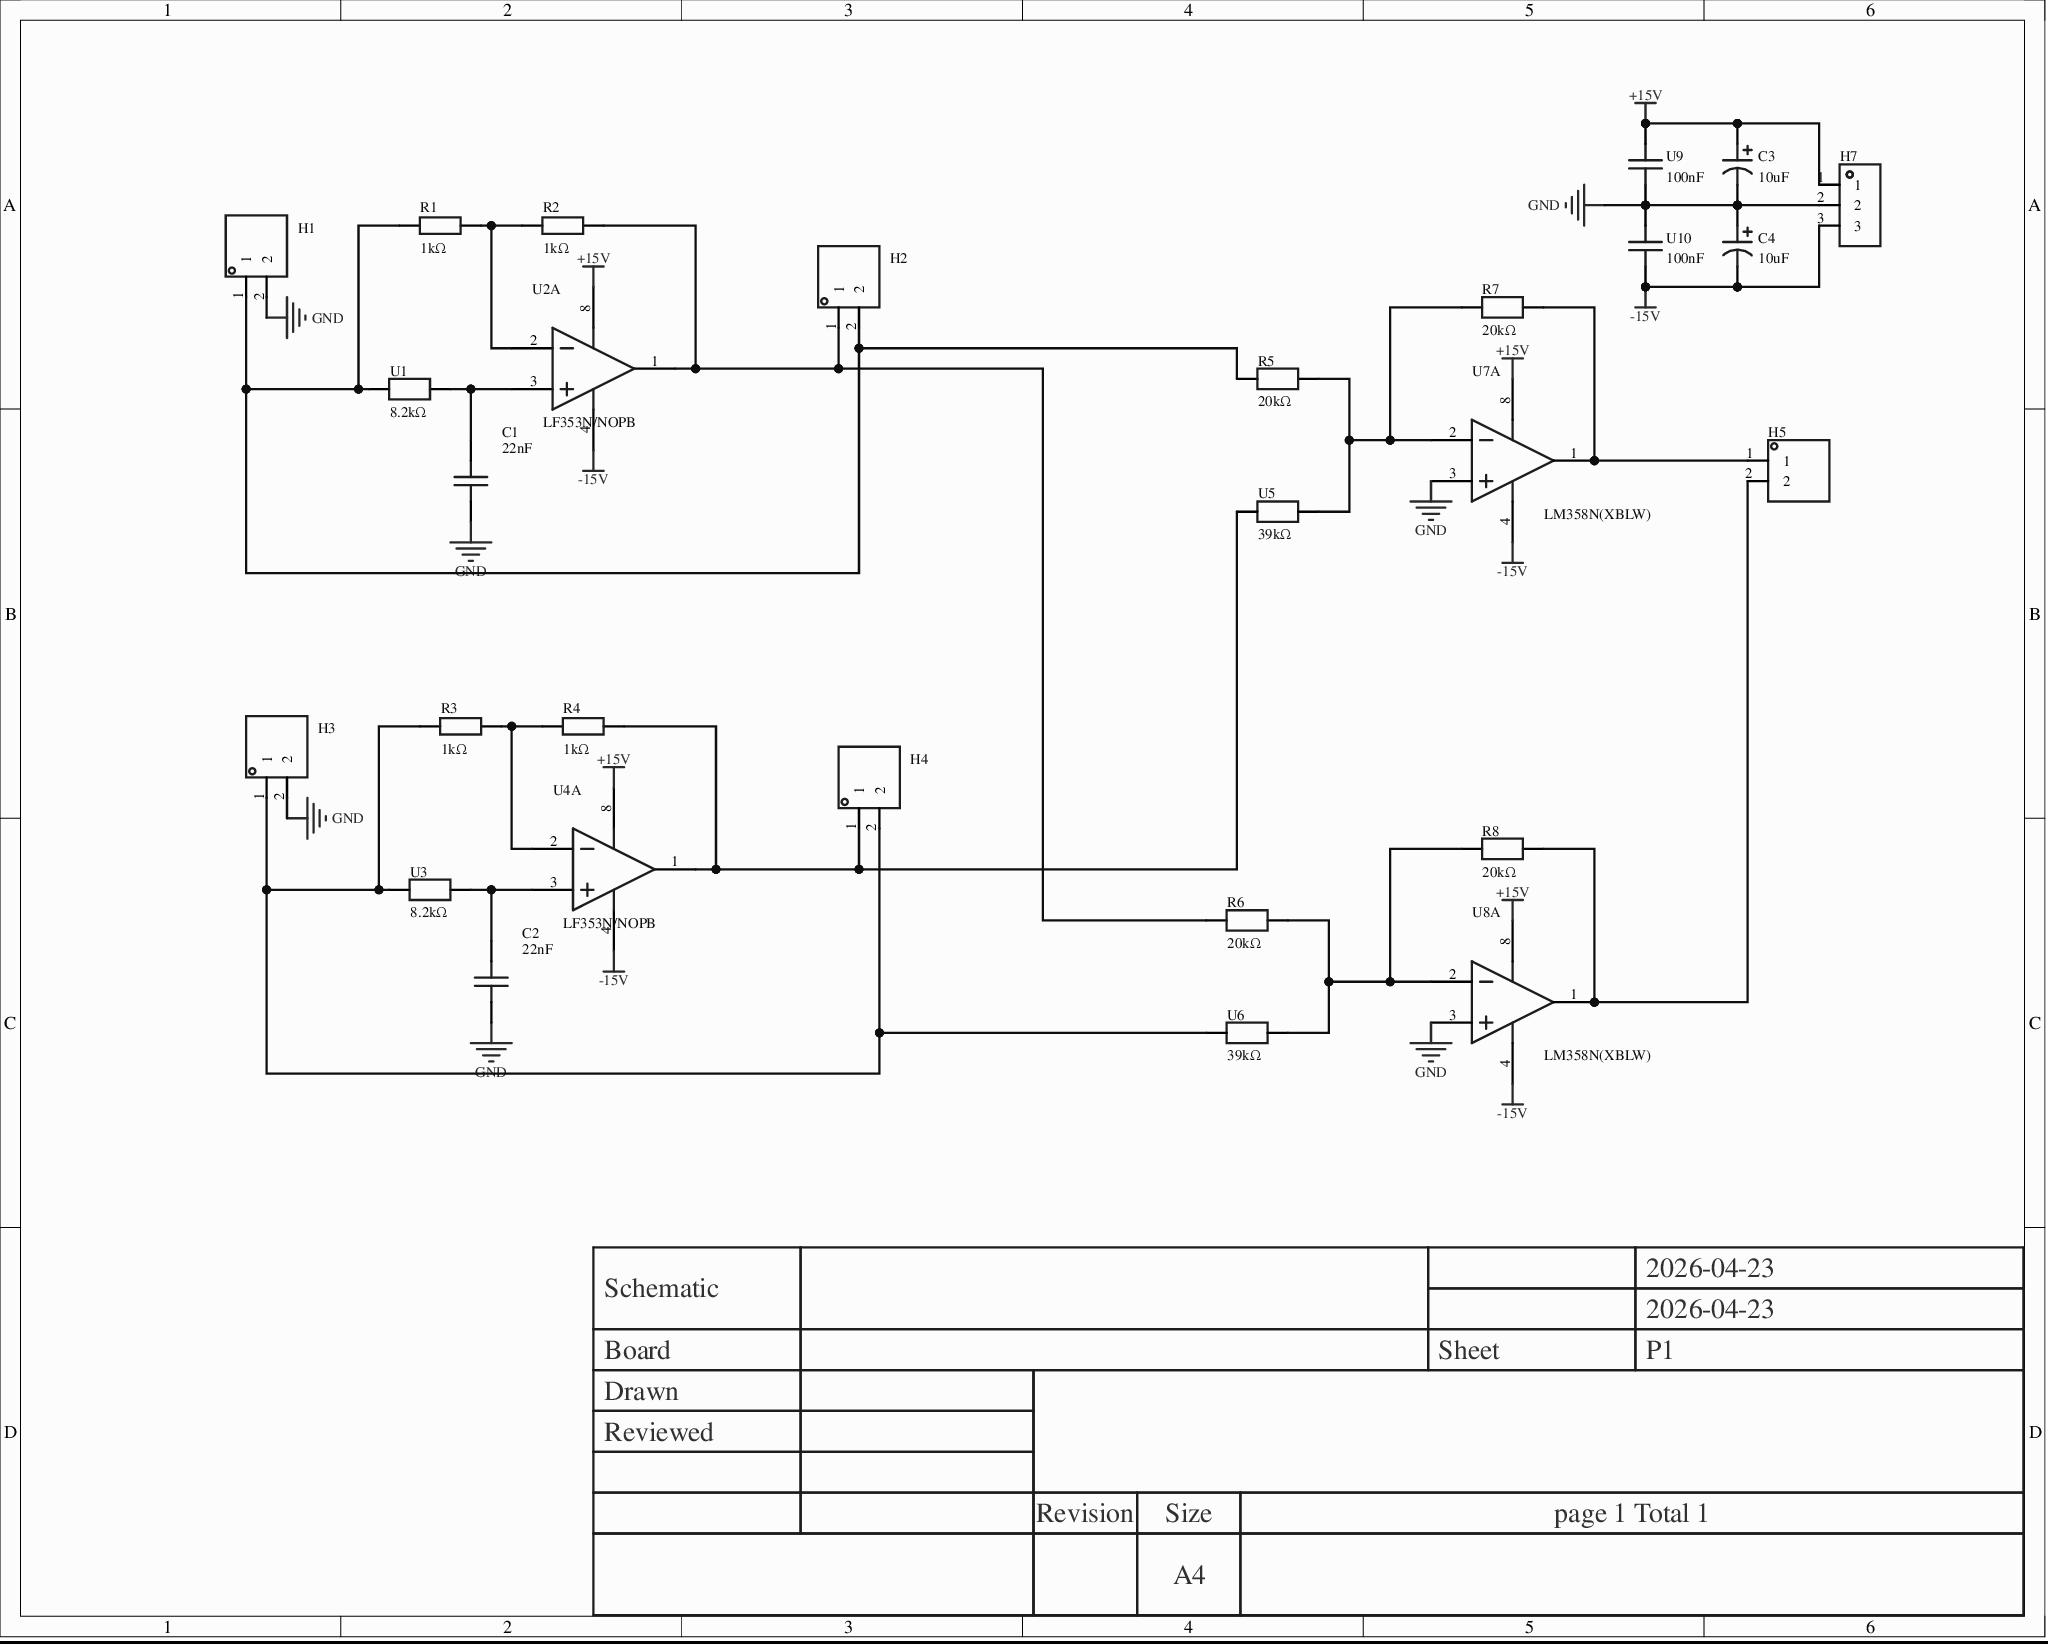
[diagram p0: MISC49900-3.schdoc]
# Altium project MISC49900-2.PrjPcb
1 sheet, 28 parts. Net scope: global (net labels, ports and power ports of the same name join across sheets).
Board file: MISC49900.pcbdoc

## Sheet MISC49900-3.schdoc
size 254 x 203 mm; Version: V1.0; @Project Name: MISC49900; @Update Date: 2026-04-26; @Create Date: 2026-04-26; @Board Name: MISC49900; @Create Time: 22:45:20; @Page Count: 1; @Page No: 1; @Schematic Name: MISC49900; @Update Time: 22:45:20; Size: A4

### Parts
C1  22nF  [CAP-TH_L12.0-W4.5-P10.00-D1.0]
C2  22nF  [CAP-TH_L12.0-W4.5-P10.00-D1.0]
C3  10uF  [CAP-TH_BD5.0-P2.00-D0.8-FD-10UF50VC110GL]
C4  10uF  [CAP-TH_BD5.0-P2.00-D0.8-FD-10UF50VC110GL]
H1  (no value)  [HDR-TH_2P-P2.54-V-M-1]
H2  (no value)  [HDR-TH_2P-P2.54-V-M-1]
H3  (no value)  [HDR-TH_2P-P2.54-V-M-1]
H4  (no value)  [HDR-TH_2P-P2.54-V-M-1]
H5  (no value)  [HDR-TH_2P-P2.54-V-M-1]
H7  (no value)  [HDR-TH_3P-P2.54-V-M]
R1  1kΩ  [RES-TH_BD2.5-L6.5-P10.50-D0.6]
R2  1kΩ  [RES-TH_BD2.5-L6.5-P10.50-D0.6]
R3  1kΩ  [RES-TH_BD2.5-L6.5-P10.50-D0.6]
R4  1kΩ  [RES-TH_BD2.5-L6.5-P10.50-D0.6]
R5  20kΩ  [RES-TH_BD2.4-L6.3-P10.30-D0.6]
R6  20kΩ  [RES-TH_BD2.4-L6.3-P10.30-D0.6]
R7  20kΩ  [RES-TH_BD2.4-L6.3-P10.30-D0.6]
R8  20kΩ  [RES-TH_BD2.4-L6.3-P10.30-D0.6]
U1  8.2kΩ  [RES-TH_BD2.7-L6.2-P10.20-D0.4]
U2  LF353N/NOPB  [PDIP-8_L9.6-W6.4-P2.54-LS7.6-BL]  (part A of 2)
U3  8.2kΩ  [RES-TH_BD2.7-L6.2-P10.20-D0.4]
U4  LF353N/NOPB  [PDIP-8_L9.6-W6.4-P2.54-LS7.6-BL]  (part A of 2)
U5  39kΩ  [RES-TH_BD2.4-L6.3-P10.30-D0.6]
U6  39kΩ  [RES-TH_BD2.4-L6.3-P10.30-D0.6]
U7  LM358N(XBLW)  [PDIP-8_L9.3-W6.4-P2.54-LS7.6-BL]  (part A of 2)
U8  LM358N(XBLW)  [PDIP-8_L9.3-W6.4-P2.54-LS7.6-BL]  (part A of 2)
U9  100nF  [CAP-TH_L5.0-W2.5-P5.00-D1.0]
U10  100nF  [CAP-TH_L5.0-W2.5-P5.00-D1.0]

### Nets
+15V: C3.1 H7.1 U2.8(VCC) U4.8(VCC) U7.8(V+) U8.8(V+) U9.1
-15V: C4.2 H7.3 U2.4(VEE) U4.4(VEE) U7.4(V-) U8.4(V-) U10.2
GND: C1.1 C2.1 C3.2 C4.1 H1.2 H3.2 H7.2 U7.3(IN_A+) U8.3(IN_A+) U9.2 U10.1
NetC1_2: C1.2 U1.2 U2.3(INA+)
NetC2_2: C2.2 U3.2 U4.3(INA+)
NetH1_1: H1.1 H2.2 R1.1 R5.1 U1.1
NetH2_1: H2.1 R2.2 R6.1 U2.1(OUTA)
NetH3_1: H3.1 H4.2 R3.1 U3.1 U6.1
NetH4_1: H4.1 R4.2 U4.1(OUTA) U5.1
NetH5_1: H5.1 R7.2 U7.1(OUT_A)
NetH5_2: H5.2 R8.2 U8.1(OUT_A)
NetR1_2: R1.2 R2.1 U2.2(INA-)
NetR3_2: R3.2 R4.1 U4.2(INA-)
NetR5_2: R5.2 R7.1 U5.2 U7.2(IN_A-)
NetR6_2: R6.2 R8.1 U6.2 U8.2(IN_A-)

### Notes on the sheet
- 2026-04-23
- Schematic
- Board
- Sheet
- P1
- Drawn
- Reviewed
- Revision
- Size
- A4
- page 1 Total 1

### Library data of the parts
C1 C2 = KP223J2J1001: component KP223J2J1001; capacitance: 22nF; tolerance: ±5%; rated voltage: 630V; operating temperature: -40℃~+100℃;; Manufacturer: KYET(科雅); AddInBom: yes; ModelId: 5745697730bf4b0891de41ab4d2b5a300819f05c4eef4c71ace90d822a990e87; ModelName: CAP-TH_L12.0-W4.5-H10.0-P10.0; ModelTransform: 472.44,177.165,0,0,0,0,0,0,-137.795; Device: KP223J2J1001; Symbol: KP223J2J1001; FootprintName: CAP-TH_L12.0-W4.5-P10.00-D1.0; LCSC Part Name: 22nF ±5% 630V; SupplierPart: C390074; ManufacturerPart: KP223J2J1001; Supplier Footprint: 插件,P=10mm; JLCPCB Part Class: Extended Part; Datasheet: example.com/datasheet/KP223J2J1001/366157.html; Supplier: LCSC; ConvertToPcb: yes; Value: 22nF; Tolerance: ±5%; Voltage Rating: 630V; Operating Temperature: -40℃~+100℃
C3 C4 = 10UF50VC110GL: component 10UF50VC110GL; capacitance: 10uF; tolerance: ±20%; rated voltage: 50V; ripple current: 120mA@100KHz; equivalent series resistance (ESR): 1.6Ω;; Manufacturer: Econd(米朗电子); AddInBom: yes; Pin Spacing: 2mm; Lifetime: 5000hrs@105℃; Symbol: 10UF50VC110GL; Device: 10UF50VC110GL; LCSC Part Name: 10uF ±20% 50V; SupplierPart: C46867109; ManufacturerPart: 10UF50VC110GL; Supplier Footprint: 插件,D5xL11mm; JLCPCB Part Class: Extended Part; Datasheet: example.com/datasheet/10UF50VC110GL/49031974.html; Supplier: LCSC; ConvertToPcb: yes; FootprintName: CAP-TH_BD5.0-P2.00-D0.8-FD-10UF50VC110GL; Value: 10uF; Tolerance: ±20%; Voltage Rating: 50V; Ripple Current: 120mA@100KHz; Equivalent Series Resistance(ESR): 1.6Ω; Diameter: 5mm; Height - Seated (Max): 11mm; Operating Temperature: -40℃~+105℃
H1-H5 = HDR-M_2.54_1x2P: Symbol: 210S-1*2P L=11.6MMGold-plated black; ConvertToPcb: yes; ModelId: 79b2e9f2d70a4d68a1b7098f27c6d4c50819f05c4eef4c71ace90d822a990e87; ModelName: HDR-M-2.54_1x2; ModelTransform: 200,100,0,0,0,0,0,0,-118.11; Device: HDR-M_2.54_1x2P; FootprintName: HDR-TH_2P-P2.54-V-M-1; AddInBom: yes; SupplierPart: C124375; Supplier Footprint: 插件
H7 = HDR-M_2.54_1x3P: AddInBom: yes; ModelId: bb473b6d38ff42a99216a4fcdbdcc4cb0819f05c4eef4c71ace90d822a990e87; ModelName: HDR-TH_3P-P2.54-M-LI-1X3P; ModelTransform: 300.03877,100,0,0,0,0,0,0,-118.11; Device: HDR-M_2.54_1x3P; Symbol: HDR-M_2.54_1x3P; FootprintName: HDR-TH_3P-P2.54-V-M; ConvertToPcb: yes; SupplierPart: C2937625; Supplier Footprint: 插件
R1-R4 = MFR0W4F1001A50: component MFR0W4F1001A50; resistor type: metal film resistor; resistance: 1kΩ; tolerance: ±1%; power: 250mW; temperature coefficient: ±50ppm/℃;; Manufacturer: UNI-ROYAL(厚声); AddInBom: yes; Voltage-Supply(Max): 250V; ModelId: 8e6c7ee8323443d1ab8f0504b6353c8c0819f05c4eef4c71ace90d822a990e87; ModelName: RES-TH_D2.3-L6.5-P10.50; ModelTransform: 431.1015,91.3384,0,0,0,0,0.197,0,-137.795; Device: MFR0W4F1001A50; Symbol: MFR0W4F1001A50; FootprintName: RES-TH_BD2.5-L6.5-P10.50-D0.6; LCSC Part Name: 1kΩ ±1% 250mW 金属膜电阻 铜脚，圆柱状直插; SupplierPart: C57435; ManufacturerPart: MFR0W4F1001A50; Supplier Footprint: 插件,D2.2xL6.5mm; JLCPCB Part Class: Extended Part; Datasheet: example.com/20191012/C436293_8820AA14BC71FA35E551C06C441482A0.pdf; Supplier: LCSC; ConvertToPcb: yes; Type: Metal film resistor; Value: 1kΩ; Tolerance: ±1%; Power(Watts): 250mW; Temperature Coefficient: ±50ppm/℃
R5 = RN 1/4W 20K F T/B A1: 电阻类型:金属膜电阻;阻值:20kΩ;精度:±1%;功率:250mW;温度系数:±50ppm/℃;; Manufacturer: Tyohm(幸亚电阻); AddInBom: yes; Tolerance: ±1%; Voltage-Supply(Max): 250V; Power(Watts): 250mW; Description: resistor type: metal film resistor; resistance: 20kΩ; tolerance: ±1%; power: 250mW; temperature coefficient: ±50ppm/℃;; ModelId: 463263665006444ab7a47bd11b0cf9560819f05c4eef4c71ace90d822a990e87; ModelTransform: 427.165,94.32816,0,0,0,0,0,0,-196.85; Device: RN 1/4W 20K F T/B A1; Symbol: RN 1/4W 20K F T/B A1; FootprintName: RES-TH_BD2.4-L6.3-P10.30-D0.6; LCSC Part Name: 20kΩ ±1% 250mW 金属膜电阻; SupplierPart: C410662; ManufacturerPart: RN 1/4W 20K F T/B A1; Supplier Footprint: 插件,D2.4xL6.4mm; JLCPCB Part Class: Extended Part; Datasheet: example.com/datasheet/RN%25201%252F4W%252020K%2520F%2520T%252FB%2520A1/401583.html; Supplier: LCSC; ConvertToPcb: yes; Type: Metal film resistor; Value: 20kΩ; Temperature Coefficient: ±50ppm/℃; Operating Temperature: -55℃~+125℃; ModelName: RES-TH_BD2.4-L6.3-P10.30-D0.6
R6-R8 = RN 1/4W 20K F T/B A1: resistor type: metal film resistor; resistance: 20kΩ; tolerance: ±1%; power: 250mW; temperature coefficient: ±50ppm/℃;; Manufacturer: Tyohm(幸亚电阻); AddInBom: yes; Voltage-Supply(Max): 250V; ModelId: 463263665006444ab7a47bd11b0cf9560819f05c4eef4c71ace90d822a990e87; ModelTransform: 427.165,94.32816,0,0,0,0,0,0,-196.85; Device: RN 1/4W 20K F T/B A1; Symbol: RN 1/4W 20K F T/B A1; FootprintName: RES-TH_BD2.4-L6.3-P10.30-D0.6; LCSC Part Name: 20kΩ ±1% 250mW 金属膜电阻; SupplierPart: C410662; ManufacturerPart: RN 1/4W 20K F T/B A1; Supplier Footprint: 插件,D2.4xL6.4mm; JLCPCB Part Class: Extended Part; Datasheet: example.com/datasheet/RN%25201%252F4W%252020K%2520F%2520T%252FB%2520A1/401583.html; Supplier: LCSC; ConvertToPcb: yes; Type: Metal film resistor; Value: 20kΩ; Tolerance: ±1%; Power(Watts): 250mW; Temperature Coefficient: ±50ppm/℃; Operating Temperature: -55℃~+125℃; ModelName: RES-TH_BD2.4-L6.3-P10.30-D0.6
U1 U3 = MF1/4W-8K2±1%-ST52: resistor type: metal film resistor; resistance: 8.2kΩ; tolerance: ±1%; power: 250mW; temperature coefficient: ±350ppm/℃;; Manufacturer: VO(翔胜); AddInBom: yes; Overload Voltage (Max): 250V; ModelId: f91fbe0e2e6f409498f09f811e4616fe0819f05c4eef4c71ace90d822a990e87; ModelTransform: 417.322,106.221,0,0,0,0,0,0,-196.85; Device: MF1/4W-8K2±1%-ST52; Symbol: MF1/4W-8K2±1%-ST52; FootprintName: RES-TH_BD2.7-L6.2-P10.20-D0.4; LCSC Part Name: 金属膜电阻 8.2kΩ ±1% 250mW; SupplierPart: C2848599; ManufacturerPart: MF1/4W-8K2±1%-ST52; Supplier Footprint: 插件,D2.7xL6.2mm; JLCPCB Part Class: Extended Part; Datasheet: example.com/20200609/C601728_5AA4C0C8E12E11069DA2C3356F29D1F2.pdf; Supplier: LCSC; ConvertToPcb: yes; Type: Metal film resistor; Value: 8.2kΩ; Tolerance: ±1%; Power(Watts): 250mW; Temperature Coefficient: ±350ppm/℃; Operating Temperature Range: -55℃~+155℃; ModelName: RES-TH_BD2.7-L6.2-P10.20-D0.4
U2 U4 = LF353N/NOPB: component LF353N/NOPB; amplifier count: -; gain-bandwidth product (GBP): 4MHz; input bias current (Ib): 50pA; input offset voltage (Vos): 5mV; slew rate (SR): 13V/us; rail-to-rail: -;; Manufacturer: TI(德州仪器); Relevance: []; AddInBom: yes; Common Mode Rejection Ratio(CMRR): 100dB; Voltage - Supply: -18V~18V; Quiescent Current per Amplifier: 3.6mA; Input Offset Voltage Drift(Vos TC): 10uV/℃; ModelId: 5dc2af053da0476fab11ee64b9a10a940819f05c4eef4c71ace90d822a990e87; ModelName: PDIP-8_L9.6-W6.4-P2.54-LS7.62-BL; ModelTransform: 377.952,309.842,0,0,0,0,0,0,-137.795; Device: LF353N/NOPB; Symbol: LF353N/NOPB; FootprintName: PDIP-8_L9.6-W6.4-P2.54-LS7.6-BL; LCSC Part Name: LF353-N 宽带双JFET输入运算放大器; SupplierPart: C2860458; ManufacturerPart: LF353N/NOPB; Supplier Footprint: PDIP-8; JLCPCB Part Class: Extended Part; Supplier: LCSC; ConvertToPcb: yes; Number of Channels: -; Gain Bandwidth Product: 4MHz; Ib - Input Bias Current: 50pA; Vos - Input Offset Voltage: 5mV; Slew Rate: 13V/us; Rail To Rail: -; Output Type: -; Output Current: -; Operating Temperature: -
  U2: Description: amplifier count: -; gain-bandwidth product (GBP): 4MHz; input bias current (Ib): 50pA; input offset voltage (Vos): 5mV; slew rate (SR): 13V/us; rail-to-rail: -;
U5 U6 = MFR-25FRF52-39K: component MFR-25FRF52-39K; resistor type: metal film resistor; resistance: 39kΩ; tolerance: ±1%; power: 250mW; temperature coefficient: ±100ppm/℃;; Manufacturer: YAGEO(国巨); AddInBom: yes; ModelId: 463263665006444ab7a47bd11b0cf9560819f05c4eef4c71ace90d822a990e87; ModelTransform: 427.165,94.32816,0,0,0,0,0,0,-196.85; Device: MFR-25FRF52-39K; Symbol: MFR-25FRF52-39K; FootprintName: RES-TH_BD2.4-L6.3-P10.30-D0.6; LCSC Part Name: 金属膜电阻 39kΩ ±1% 250mW; SupplierPart: C1744105; ManufacturerPart: MFR-25FRF52-39K; Supplier Footprint: 插件,D2.4xL6.3mm; JLCPCB Part Class: Extended Part; Datasheet: example.com/datasheet/MFR-25FRF52-39K/1834886.html; Supplier: LCSC; ConvertToPcb: yes; Type: Metal film resistor; Value: 39kΩ; Tolerance: ±1%; Power(Watts): 250mW; Temperature Coefficient: ±100ppm/℃; Operating Temperature: -55℃~+155℃; ModelName: RES-TH_BD2.4-L6.3-P10.30-D0.6
U7 U8 = LM358N(XBLW): component LM358N(XBLW); amplifier count: 2; rail-to-rail: -; gain-bandwidth product (GBW): -; input offset voltage (Vos): 5mV; slew rate (SR): 600V/ms; input bias current (Ib): 300nA;; Manufacturer: XBLW(芯伯乐); Relevance: []; AddInBom: yes; Number of Channels: 2; Maximum Power Supply Range (Vdd-Vss): 32V; Input Offset Voltage Drift(Vos TC): 7uV/℃; Input Offset Current(Ios): 3nA; Common Mode Rejection Ratio(CMRR): 90dB; Quiescent Current: 500uA; Output Current: 40mA; Single supply: 3V~24V; Dual Supply: -12V~-1.5V; 1.5V~12V; ModelId: fe5fd42f66544692923c5fbf1ee41ec70819f05c4eef4c71ace90d822a990e87; ModelName: PDIP-8_L10.2-W5.9-H4.5-P2.54-LS7.6-BL; ModelTransform: 364.173,311.8104,0,0,0,0,0,0,-118.11; Device: LM358N(XBLW); Symbol: LM358N(XBLW); FootprintName: PDIP-8_L9.3-W6.4-P2.54-LS7.6-BL; LCSC Part Name: 低功耗双运算放大器; SupplierPart: C18723615; ManufacturerPart: LM358N(XBLW); Supplier Footprint: DIP-8; JLCPCB Part Class: Extended Part; Datasheet: example.com/datasheet/LM358N(XBLW)/19916742.html; Supplier: LCSC; ConvertToPcb: yes; Rail to Rail: -; Gain Bandwidth Product: -; Vos - Input Offset Voltage: 5mV; Slew Rate: 600V/ms; Ib - Input Bias Current: 300nA; Input Voltage Noise Density: -; Input offset current drift(Ios TC): -; Operating Temperature: 0℃~+70℃; Features: -
  U7: Description: amplifier count: 2; rail-to-rail: -; gain-bandwidth product (GBW): -; input offset voltage (Vos): 5mV; slew rate (SR): 600V/ms; input bias current (Ib): 300nA;
U9 U10 = 100nF: Symbol: 100NF_C9900015256; AddInBom: yes; ModelId: 08e3d7481fc7486bb1b263873f51e1e10819f05c4eef4c71ace90d822a990e87; ModelName: CAP-TH_BD5.0-W2.5-P5.08; ModelTransform: 224.652,98.425,0,0,0,0,-0.005,0,-137.795; Device: 100nF; LCSC Part Name: 100nF; SupplierPart: C9900015256; ManufacturerPart: 100nF; Supplier Footprint: CAP-TH_L5.0-W2.5-P5.00-D1.0; JLCPCB Part Class: Extended Part; Supplier: LCSC; ConvertToPcb: yes; FootprintName: CAP-TH_L5.0-W2.5-P5.00-D1.0